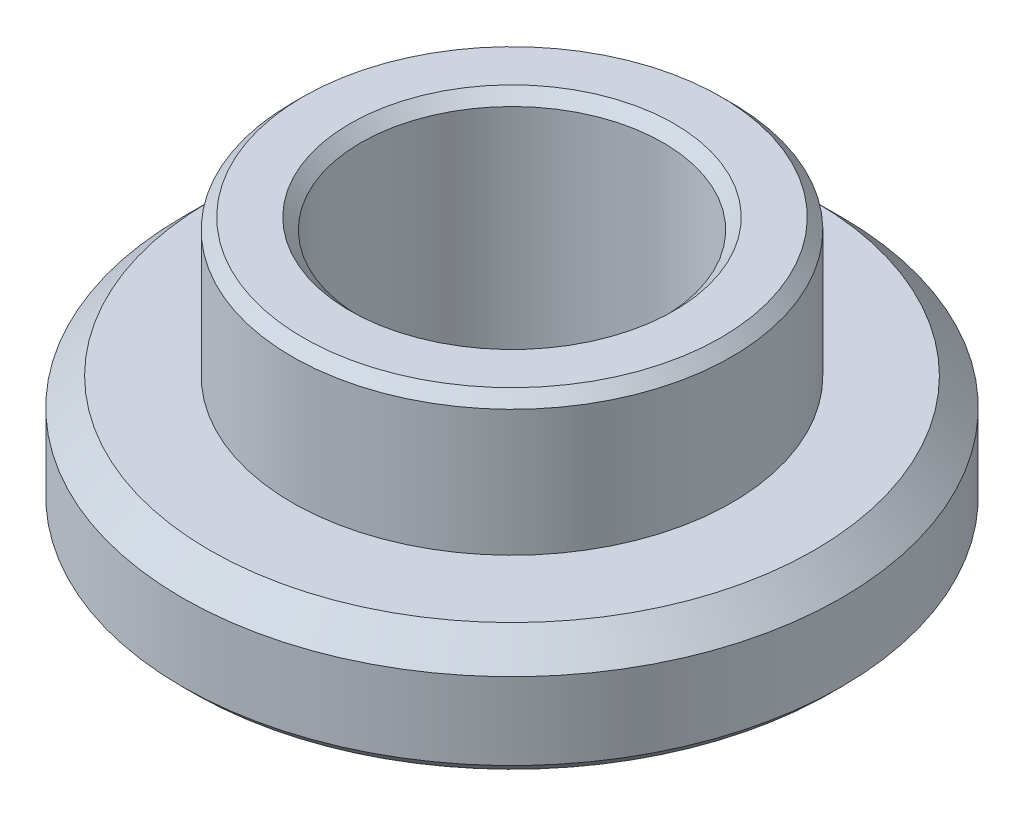
from build123d import *


with BuildPart() as part:
    # Sketch1 → Revolve1 (revolve)
    with BuildSketch(Plane.XY):
        Polygon((-29.5, 0), (-58, 0), (-60, 2), (-60, 16), (-55, 21), (-40, 21), (-40, 44), (-38, 46), (-29.5, 46), (-27.5, 44), (-27.5, 2), align=None)
    revolve(axis=Axis((0, 46, 0), (0, -1, 0)))


solid = part.part
